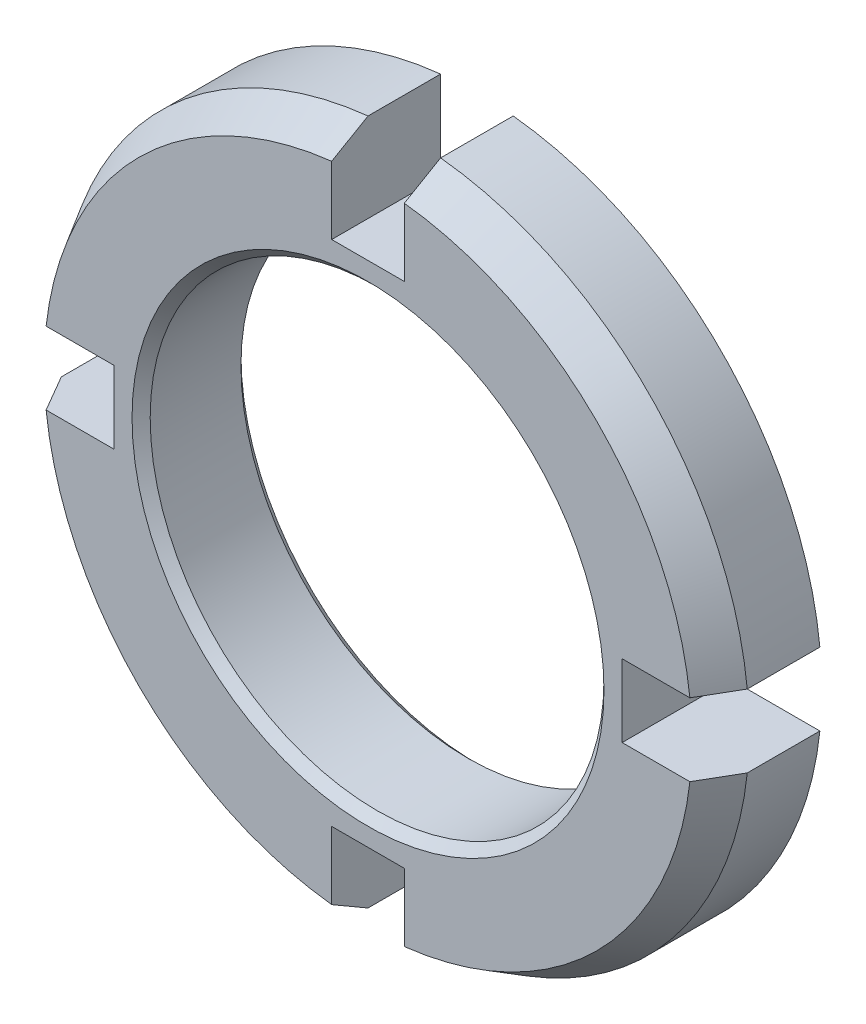
SolidWorks part; units mm, degrees
ref_plane "Front Plane" through (0, 0, 0) normal (0, 0, 1) x (1, 0, 0)
ref_plane "Top Plane" through (0, 0, 0) normal (0, 1, 0) x (1, 0, 0)
ref_plane "Right Plane" through (0, 0, 0) normal (1, 0, 0) x (0, 0, -1)
sketch "Sketch1" plane through (0, 0, 0) normal (0, 0, 1) x (1, 0, 0)
  circle A0 centre (0, 0) radius 19
  circle A1 centre (0, 0) radius 12.5
  dimension "D1" = 38
  dimension "D2" = 25
extrude "Boss-Extrude1" add sketch "Sketch1" along normal blind 6
ref_plane "Plane1" through (14, 0, 0) normal (1, 0, 0) x (0, 0, -1)
sketch "Sketch2" plane through (14, 0, 0) normal (1, 0, 0) x (0, 0, -1)
  line L0 (0, -19) -> (0, 19) construction
  line L1 (0, -2) -> (-6, -2)
  line L2 (0, -2) -> (0, 2)
  line L3 (0, 2) -> (-6, 2)
  line L4 (-6, -2) -> (-6, 2)
  line L5 (-6, 19) -> (-6, -19) construction
  line L6 (0, 0) -> (-13.2085, 0) construction
  dimension "D1" = 4
extrude "Cut-Extrude1" cut sketch "Sketch2" along normal blind 6
pattern_circular "CirPattern1" count 4 over 360 about axis through (0, 0, 0) along (0, 0, 1) of "Cut-Extrude1"
chamfer "Chamfer1" distance 0.5 angle 45 2 edges at (12.5, 0, 6) (12.5, 0, 0)
chamfer "Chamfer2" distance 2 angle 30 4 edges at (13.435, -13.435, 6) (-13.435, -13.435, 6) (13.435, 13.435, 6) (-13.435, 13.435, 6)
